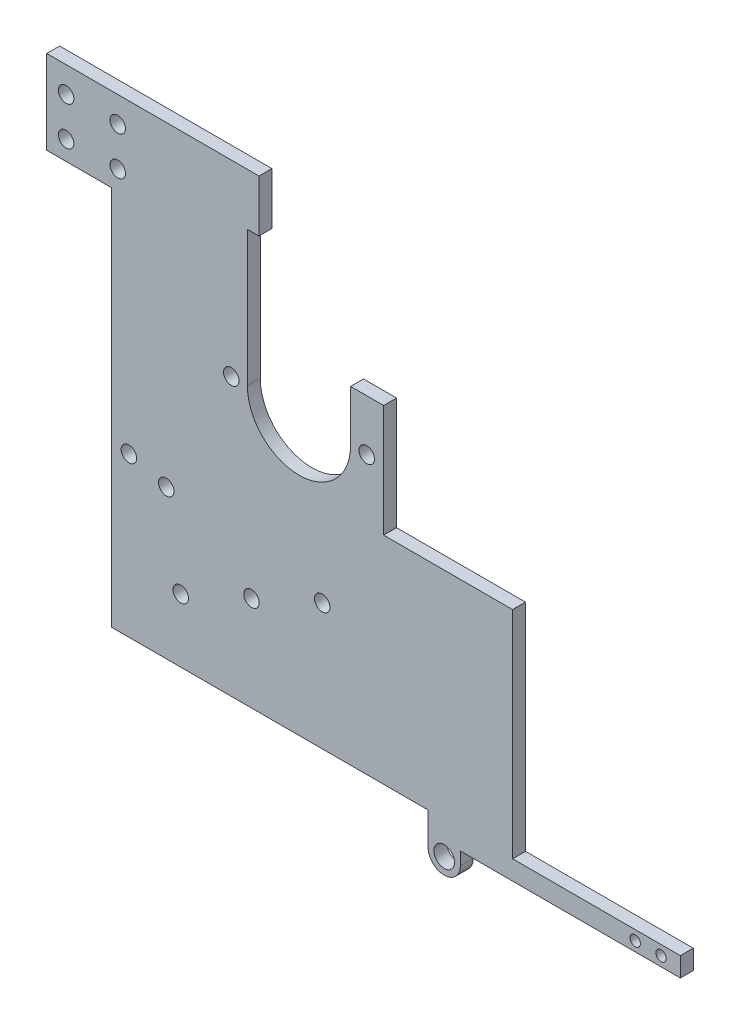
from build123d import *

# Parameters (mm, degrees)
SKETCH_1_R               = 5
SKETCH_1_R_2             = 6
EXTRUDE_1_DEPTH          = 10
SKETCH_2_R               = 6
CUT_EXTRUDE_1_DEPTH      = 10
SKETCH_3_R               = 8
SKETCH_3_R_2             = 4
EXTRUDE_2_DEPTH          = 10
CUT_EXTRUDE_3_DEPTH      = 417.865256367
CUT_EXTRUDE_3_DEPTH_BACK = 10
SKETCH_4_R               = 5
SKETCH_5_R               = 5
EXTRUDE_3_DEPTH          = 10
SKETCH_6_R               = 5
EXTRUDE_4_DEPTH          = 10
EXTRUDE_5_DEPTH          = 10


with BuildPart() as part:
    # 草图1 → 凸台-拉伸1 (new body)
    with BuildSketch(Plane.XY):
        with BuildLine():
            Line((-200.997267146, -87.263605576), (110, -87.263605576))
            Line((110, -87.263605576), (110, 0))
            Line((110, 0), (110, 79.983892276))
            Line((110, 79.983892276), (85.070632456, 79.983892276))
            Line((85.070632456, 79.983892276), (85.070632456, 49.983892276))
            ThreePointArc((85.070632456, 49.983892276), (55.070632456, 19.983892276), (25.070632456, 49.983892276))
            Line((25.070632456, 49.983892276), (25.070632456, 79.983892276))
            Line((25.070632456, 79.983892276), (10.070632456, 79.983892276))
            Line((10.070632456, 79.983892276), (10.070632456, 166.983892276))
            Line((10.070632456, 166.983892276), (-15.514893523, 166.983892276))
            Line((-15.514893523, 166.983892276), (-15.514893523, 127.416711183))
            ThreePointArc((-15.514893523, 127.416711183), (-55.514893523, 87.416711183), (-95.514893523, 127.416711183))
            Line((-95.514893523, 127.416711183), (-95.514893523, 232.416711183))
            Line((-95.514893523, 232.416711183), (-86.514893523, 232.416711183))
            Line((-86.514893523, 232.416711183), (-86.514893523, 332.416711183))
            Line((-86.514893523, 332.416711183), (-110.997267146, 332.416711183))
            Line((-110.997267146, 332.416711183), (-110.997267146, 302.681550212))
            ThreePointArc((-110.997267146, 302.681550212), (-140.997267146, 272.681550212), (-170.997267146, 302.681550212))
            Line((-170.997267146, 302.681550212), (-170.997267146, 332.681550212))
            Line((-170.997267146, 332.681550212), (-200.997267146, 332.681550212))
            Line((-200.997267146, 332.681550212), (-250.997267146, 332.681550212))
            Line((-250.997267146, 332.681550212), (-250.997267146, 212.681550212))
            Line((-250.997267146, 212.681550212), (-250.997267146, 207.681550212))
            Line((-250.997267146, 207.681550212), (-200.997267146, 207.681550212))
            Line((-200.997267146, 207.681550212), (-200.997267146, 182.681550212))
            Line((-200.997267146, 182.681550212), (-200.997267146, -44.649528276))
            Line((-200.997267146, -44.649528276), (-200.997267146, -87.263605576))
        make_face()
        with Locations((96.070632456, 49.983892276)):
            Circle(SKETCH_1_R, mode=Mode.SUBTRACT)
        with Locations((14.070632456, 49.983892276)):
            Circle(SKETCH_1_R, mode=Mode.SUBTRACT)
        with Locations((-3.014893523, 127.416711183)):
            Circle(SKETCH_1_R_2, mode=Mode.SUBTRACT)
        with Locations((-108.014893523, 127.416711183)):
            Circle(SKETCH_1_R_2, mode=Mode.SUBTRACT)
        with Locations((-99.997267146, 302.681550212)):
            Circle(SKETCH_1_R, mode=Mode.SUBTRACT)
        with Locations((-181.997266842, 302.67655009)):
            Circle(SKETCH_1_R, mode=Mode.SUBTRACT)
        with Locations((-37.523881476, 10.659198545)):
            Circle(SKETCH_1_R_2, mode=Mode.SUBTRACT)
        with Locations((-92.336608934, -13.745000039)):
            Circle(SKETCH_1_R_2, mode=Mode.SUBTRACT)
        with Locations((-147.149336393, -38.149198624)):
            Circle(SKETCH_1_R_2, mode=Mode.SUBTRACT)
        with Locations((-235.997267146, 222.681550212)):
            Circle(SKETCH_1_R_2, mode=Mode.SUBTRACT)
        with Locations((-195.999464127, 222.681550212)):
            Circle(SKETCH_1_R_2, mode=Mode.SUBTRACT)
        with Locations((-235.997267146, 252.681550212)):
            Circle(SKETCH_1_R_2, mode=Mode.SUBTRACT)
        with Locations((-195.997267146, 252.681550131)):
            Circle(SKETCH_1_R_2, mode=Mode.SUBTRACT)
    extrude(amount=EXTRUDE_1_DEPTH)

    # 草图2 → 切除-拉伸1 (cut)
    with BuildSketch(Plane.XY.offset(10)):
        with Locations((-158.358654267, 28.055066971)):
            Circle(SKETCH_2_R)
        with Locations((-187.336429056, 35.819638324)):
            Circle(SKETCH_2_R)
    extrude(amount=-CUT_EXTRUDE_1_DEPTH, mode=Mode.SUBTRACT)

    # 草图3 → 凸台-拉伸2 (add)
    with BuildSketch(Plane.XY.offset(10)):
        with BuildLine():
            Line((110, -87.263605576), (62, -87.263605576))
            Line((62, -87.263605576), (44.5, -87.263605576))
            Line((44.5, -87.263605576), (44.5, -112.263605576))
            ThreePointArc((44.5, -112.263605576), (57, -124.763605576), (69.5, -112.263605576))
            Line((69.5, -112.263605576), (69.5, -102.263605576))
            Line((69.5, -102.263605576), (240, -102.263605576))
            Line((240, -102.263605576), (240, -87.263605576))
            Line((240, -87.263605576), (110, -87.263605576))
        make_face()
        with Locations((57, -112.263605576)):
            Circle(SKETCH_3_R, mode=Mode.SUBTRACT)
        with Locations((225, -94.763605576)):
            Circle(SKETCH_3_R_2, mode=Mode.SUBTRACT)
        with Locations((205, -94.763605576)):
            Circle(SKETCH_3_R_2, mode=Mode.SUBTRACT)
    extrude(amount=-EXTRUDE_2_DEPTH)

    # 草图4 → 切除-拉伸3 (cut, two sides: drawn at the far end of the back side and taken through both)
    # profile 1 of 2: a face of its own
    with BuildSketch(Plane(origin=(0, 0, 0), x_dir=(-1, 0, 0), z_dir=(0, 0, -1)).offset(-CUT_EXTRUDE_3_DEPTH_BACK)):
        with BuildLine():
            ThreePointArc((170.997267146, 302.681550212), (162.210470582, 281.468346776), (140.997267146, 272.681550212))
            Line((140.997267146, 272.681550212), (250.997267146, 272.681550212))
            Line((250.997267146, 272.681550212), (250.997267146, 332.681550212))
            Line((250.997267146, 332.681550212), (170.997267146, 332.681550212))
            Line((170.997267146, 332.681550212), (170.997267146, 302.681550212))
        make_face()
        with Locations((181.997266842, 302.67655009)):
            Circle(SKETCH_4_R, mode=Mode.SUBTRACT)
    # profile 2 of 2: a face of its own
    with BuildSketch(Plane(origin=(0, 0, 0), x_dir=(-1, 0, 0), z_dir=(0, 0, -1)).offset(-CUT_EXTRUDE_3_DEPTH_BACK)):
        with BuildLine():
            Line((86.514893523, 272.681550212), (140.997267146, 272.681550212))
            ThreePointArc((140.997267146, 272.681550212), (119.784063711, 281.468346776), (110.997267146, 302.681550212))
            Line((110.997267146, 302.681550212), (110.997267146, 332.416711183))
            Line((110.997267146, 332.416711183), (86.514893523, 332.416711183))
            Line((86.514893523, 332.416711183), (86.514893523, 272.681550212))
        make_face()
        with Locations((99.997267146, 302.681550212)):
            Circle(SKETCH_4_R, mode=Mode.SUBTRACT)
    extrude(amount=CUT_EXTRUDE_3_DEPTH + CUT_EXTRUDE_3_DEPTH_BACK, mode=Mode.SUBTRACT)

    # 草图5 → 凸台-拉伸3 (add)
    with BuildSketch(Plane(origin=(0, 0, 0), x_dir=(-1, 0, 0), z_dir=(0, 0, -1))):
        with Locations((-96.070632456, 49.983892276)):
            Circle(SKETCH_5_R)
    extrude(amount=-EXTRUDE_3_DEPTH)

    # 草图6 → 凸台-拉伸4 (add)
    with BuildSketch(Plane(origin=(0, 0, 0), x_dir=(-1, 0, 0), z_dir=(0, 0, -1))):
        with Locations((-14.070632456, 49.983892276)):
            Circle(SKETCH_6_R)
    extrude(amount=-EXTRUDE_4_DEPTH)

    # 草图7 → 凸台-拉伸5 (add)
    with BuildSketch(Plane(origin=(0, 0, 0), x_dir=(-1, 0, 0), z_dir=(0, 0, -1))):
        with BuildLine():
            Line((-85.070632456, 79.983892276), (-85.070632456, 49.983892276))
            ThreePointArc((-85.070632456, 49.983892276), (-55.070632456, 19.983892276), (-25.070632456, 49.983892276))
            Line((-25.070632456, 49.983892276), (-25.070632456, 79.983892276))
            Line((-25.070632456, 79.983892276), (-85.070632456, 79.983892276))
        make_face()
    extrude(amount=-EXTRUDE_5_DEPTH)


solid = part.part
